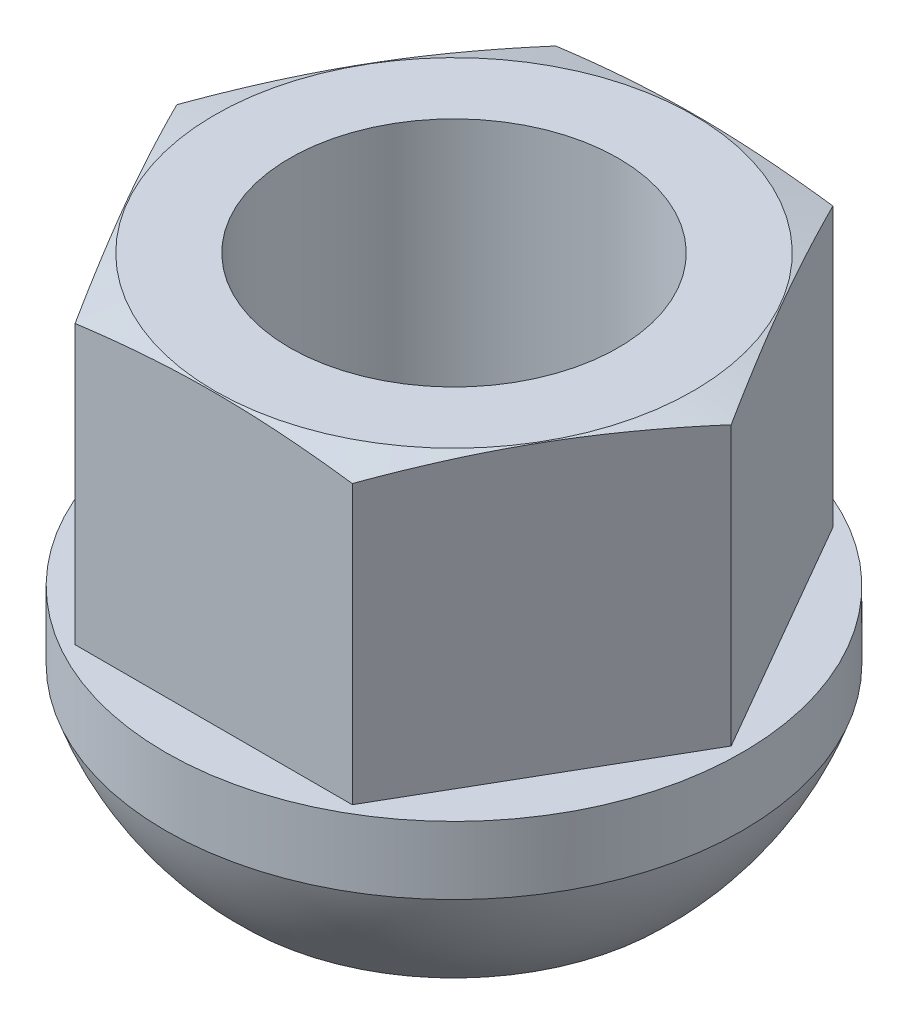
SolidWorks part; units mm, degrees
material "普通碳钢"
ref_plane "前视" through (0, 0, 0) normal (0, 0, 1) x (1, 0, 0)
ref_plane "上视" through (0, 0, 0) normal (0, 1, 0) x (1, 0, 0)
ref_plane "右视" through (0, 0, 0) normal (1, 0, 0) x (0, 0, -1)
sketch "草图1" plane through (0, 0, 0) normal (0, 0, 1) x (1, 0, 0)
  line L0 (-40.3875, 0) -> (44.55, 0) construction
  line L1 (0, 29.8688) -> (0, -34.3688) construction
  line L2 (-18, 7.7736) -> (-18, 30)
  line L3 (-18, 30) -> (-10, 30)
  line L6 (-13, 0) -> (-11.25, 0)
  line L7 (-11.25, 0) -> (-11.25, 4)
  line L8 (-11.25, 4) -> (-10, 5.2)
  line L9 (-10, 5.2) -> (-10, 30)
  arc A0 (-18, 7.7736) -> (-13, 0) centre (0, 13.8564) ccw
  dimension "D4" = 38
  dimension "D1" = 22.5
  dimension "D2" = 26
  dimension "D3" = 36
  dimension "D5" = 4
  dimension "D6" = 30
  dimension "D7" = 1.2
  dimension "D8" = 10
revolve "旋转1" add sketch "草图1" angle 360 about L1
hole_wizard "M22x1.5 螺纹孔1" positions "草图3" profile "草图2" tap size "M22x1.5" standard "GB" end condition through all
sketch "草图3" plane through (0, 30, 0) normal (0, 1, 0) x (1, 0, 0)
  point P0 (0, 0)
sketch "草图2" plane through (0, 30, 0) normal (1, 0, 0) x (0, 0, 1)
  line L0 (0, 0) -> (0, 30)
  line L1 (0, 30) -> (10.25, 30)
  line L2 (10.25, 30) -> (10.25, 0)
  line L5 (10.25, 0) -> (0, 0)
  line L11 (0, -6.35) -> (0, 107.95) construction
  dimension "通孔螺纹孔钻头直径" = 20.5
  dimension "通孔螺纹孔钻头深度" = 30
cosmetic thread "孔螺蚊线1" parameters "D2"=22
sketch "草图4" plane through (0, 30, 0) normal (0, 1, 0) x (1, 0, 0)
  line L0 (-8.65, 15) -> (8.65, 15)
  line L1 (0, -50) -> (0, 50) construction
  line L2 (-50, 0) -> (50, 0) construction
  line L3 (-8.65, 15) -> (-17.3, 0)
  line L4 (8.65, 15) -> (17.3, 0)
  line L5 (-8.65, -15) -> (8.65, -15)
  line L6 (-8.65, -15) -> (-17.3, 0)
  line L7 (8.65, -15) -> (17.3, 0)
  dimension "D1" = 17.3
  dimension "D2" = 8.65
  dimension "D3" = 15
  dimension "D4" = 34.6
  dimension "D5" = 17.3
  dimension "D6" = 15
extrude "切除-拉伸1" cut sketch "草图4" against normal blind 18 flip side to cut
sketch "草图6" plane through (0, 0, 0) normal (1, 0, 0) x (0, 0, -1)
  line L0 (6.1629, 32.3486) -> (24.1476, 27.5297)
  line L7 (0, 30) -> (15, 30) construction
  line L8 (24.1476, 27.5297) -> (24.1476, 34)
  line L9 (24.1476, 34) -> (6.1629, 34)
  line L10 (6.1629, 34) -> (6.1629, 32.3486)
  dimension "D2" = 15
revolve "切除-旋转8" cut sketch "草图6" angle 360
